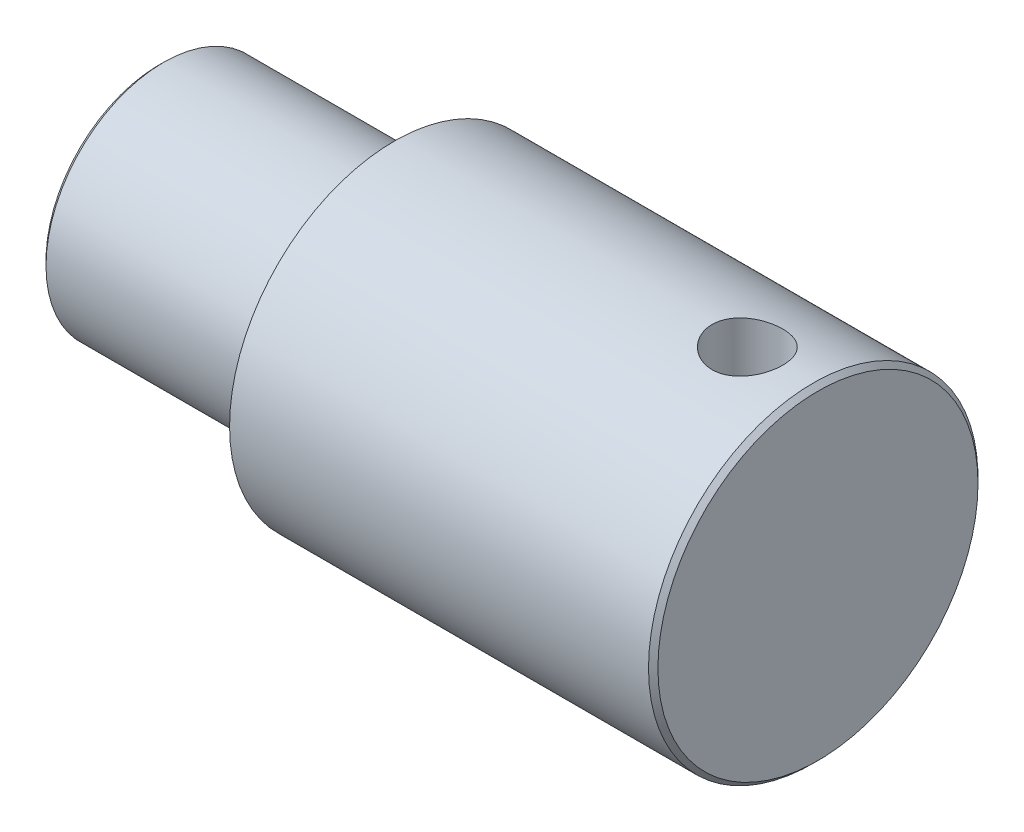
from build123d import *

# Parameters (mm, degrees)
CHAMFER1_SIZE           = 0.2
CUT_EXTRUDE2_DEPTH      = 30.69848481
CUT_EXTRUDE2_DEPTH_BACK = 30.69848481
SKETCH3_R               = 1.5
CHAMFER2_SIZE           = 0.2


with BuildPart() as part:
    # Sketch1 → Revolve1 (revolve)
    with BuildSketch(Plane.XY, mode=Mode.PRIVATE) as revolve1_sk:
        Polygon((0, 0), (0, 5), (10, 5), (10, 7), (28, 7), (28, 0), align=None)
    revolve(revolve1_sk.sketch.rotate(Axis((0, 0, 0), (1, 0, 0)), 90), axis=Axis((0, 0, 0), (1, 0, 0)))

    # Chamfer1
    chamfer1_edges = [part.edges().sort_by_distance(p)[0] for p in [
        (0, 0, -5),
    ]]
    chamfer(chamfer1_edges, length=CHAMFER1_SIZE)

    # Sketch3 → Cut-Extrude2 (cut, two sides: drawn at the far end of the back side and taken through both)
    with BuildSketch(Plane(origin=(0, 0, 0), x_dir=(1, 0, 0), z_dir=(0, 1, 0)).offset(-CUT_EXTRUDE2_DEPTH_BACK)):
        with Locations(Location((25, 0, 0), (0, 0, 270))):
            Circle(SKETCH3_R)
    extrude(amount=CUT_EXTRUDE2_DEPTH + CUT_EXTRUDE2_DEPTH_BACK, mode=Mode.SUBTRACT)

    # Chamfer2
    chamfer2_edges = [part.edges().sort_by_distance(p)[0] for p in [
        (28, 0, -7),
    ]]
    chamfer(chamfer2_edges, length=CHAMFER2_SIZE)


solid = part.part
